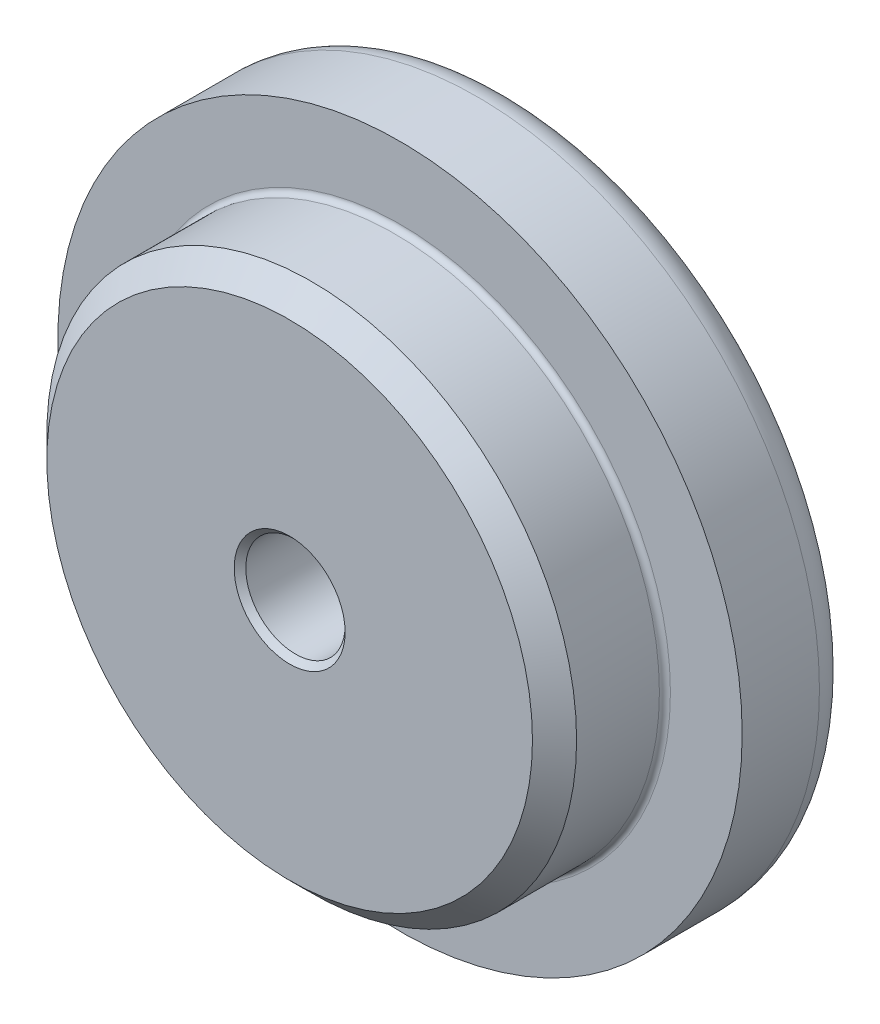
SolidWorks part; units mm, degrees
material "铝青铜"
ref_plane "前视基准面" through (0, 0, 0) normal (0, 0, 1) x (1, 0, 0)
ref_plane "上视基准面" through (0, 0, 0) normal (0, 1, 0) x (1, 0, 0)
ref_plane "右视基准面" through (0, 0, 0) normal (1, 0, 0) x (0, 0, -1)
sketch "草图1" plane through (0, 0, 0) normal (0, 0, 1) x (1, 0, 0)
  circle A0 centre (0, 0) radius 31
  dimension "D1" = 62
extrude "凸台-拉伸1" add sketch "草图1" along normal blind 10
sketch "草图2" plane through (0, 0, 10) normal (0, 0, 1) x (1, 0, 0)
  circle A0 centre (0, 0) radius 24
  dimension "D1" = 48
extrude "凸台-拉伸2" add sketch "草图2" along normal blind 10
cosmetic thread "装饰螺纹线1" parameters "D1"=9.5, "D2"=42.587
chamfer "倒角1" distance 2 angle 45 1 edges at (24, 0, 20)
fillet "圆角1" radius 3 1 edges at (31, 0, 0)
hole_wizard "M10x1.0 螺纹孔1" positions "3D草图1" profile "草图3" tap size "M10x1.0" standard "GB"
sketch3d "3D草图1"
  circle A0 centre (0, 0, 20) radius 22 construction
  point P0 (0, 0, 20)
  point P5 (0, 0, 42)
sketch "草图3" plane through (0, 0, 20) normal (1, 0, 0) x (0, -1, 0)
  line L0 (0, 0) -> (0, 27.7039)
  line L1 (0, 27.7039) -> (4.5, 25)
  line L2 (4.5, 25) -> (4.5, 0.525)
  line L3 (4.5, 0.525) -> (5.025, 0)
  line L5 (5.025, 0) -> (0, 0)
  line L6 (-4.5, 0.525) -> (-5.025, 0) construction
  line L10 (0, 27.7039) -> (-4.5, 25) construction
  line L11 (0, -6.35) -> (0, 107.95) construction
  dimension "螺纹孔钻头直径" = 9
  dimension "螺纹孔钻头深度" = 25
  dimension "近端锥形沉头孔直径" = 10.05
  dimension "近端锥形沉头孔角度" = 90
  dimension "导头角度" = 118
cosmetic thread "孔螺蚊线1" parameters "D1"=20, "D2"=10
sketch "草图4" plane through (0, 0, 0) normal (0, 0, -1) x (-1, 0, 0)
  line L0 (0, -25) -> (0, 25) construction
  line L1 (-3, -25) -> (-3, 25)
  line L2 (3, -25) -> (3, 25)
  arc A0 (-3, -25) -> (3, -25) centre (0, -25) ccw
  arc A1 (3, 25) -> (-3, 25) centre (0, 25) ccw
  point P2 (0, 0)
  dimension "D1" = 3
  dimension "D2" = 50
extrude "切除-拉伸1" cut sketch "草图4" against normal blind 1
sketch "草图5" plane through (0, 0, 0) normal (0, 0, -1) x (-1, 0, 0)
  line L0 (-25, 0) -> (25, 0) construction
  line L1 (-25, 3) -> (25, 3)
  line L2 (-25, -3) -> (25, -3)
  arc A0 (-25, 3) -> (-25, -3) centre (-25, 0) ccw
  arc A1 (25, -3) -> (25, 3) centre (25, 0) ccw
  point P2 (0, 0)
  dimension "D1" = 3
  dimension "D2" = 50
extrude "切除-拉伸2" cut sketch "草图5" against normal blind 1
fillet "圆角2" radius 0.5 1 edges at (24, 0, 10)
